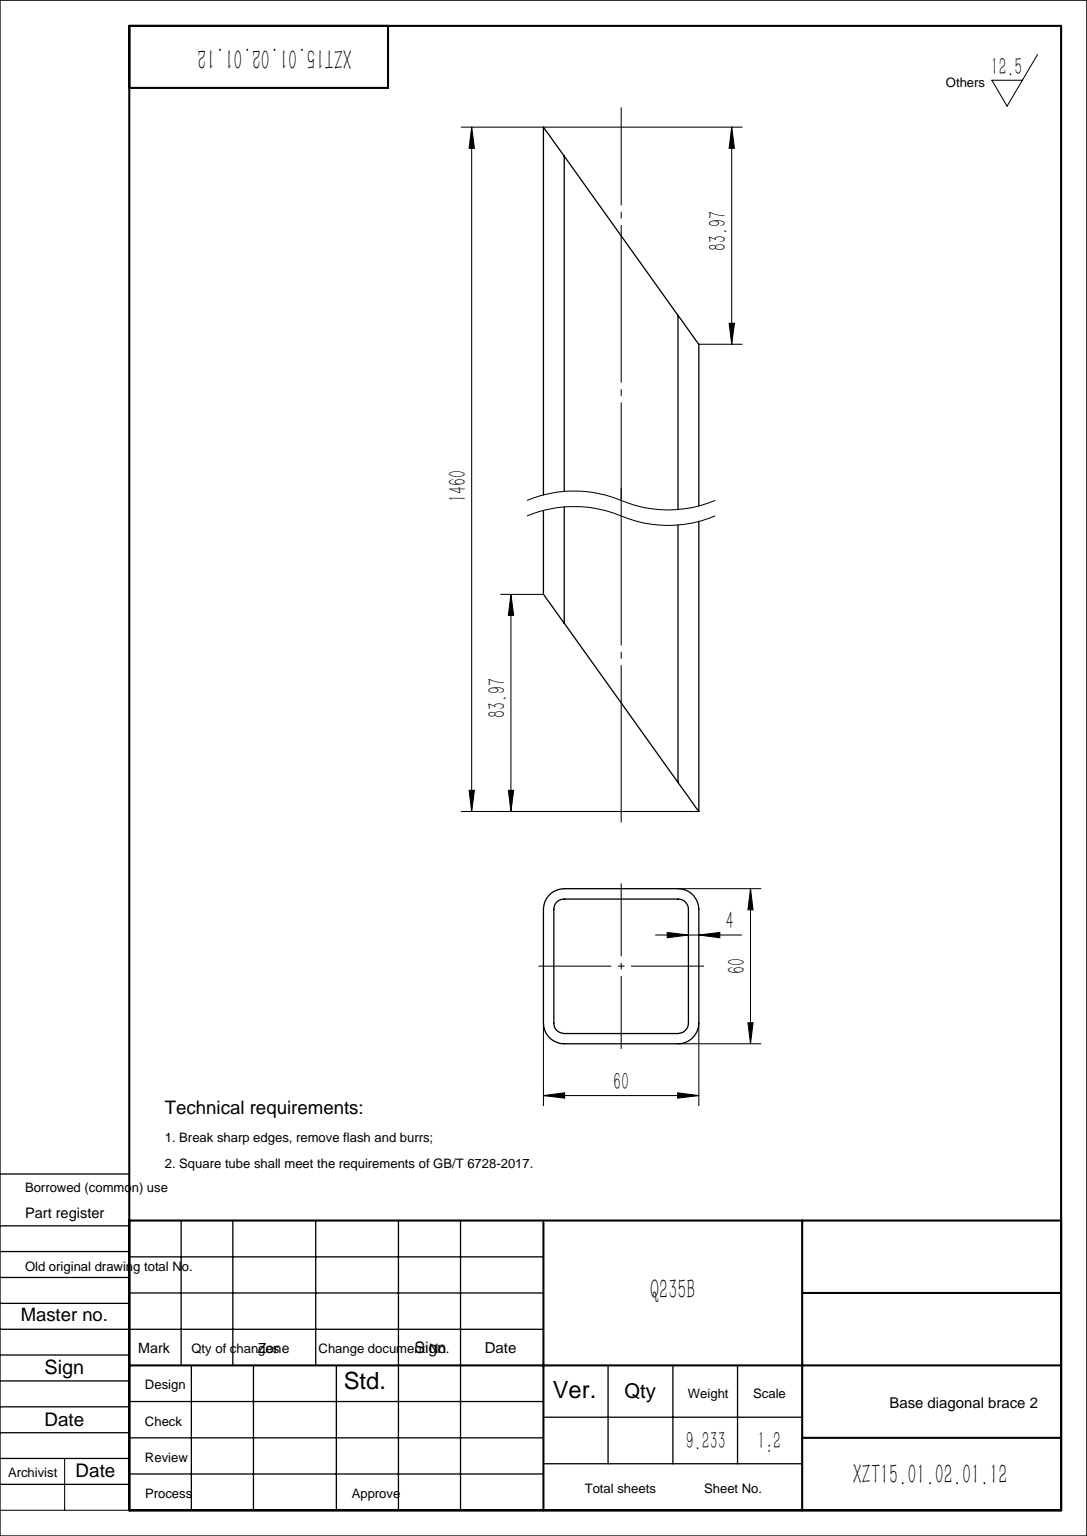
SolidWorks part; units mm, degrees
material "Q235B"
ref_plane "Front Plane" through (0, 0, 0) normal (0, 0, 1) x (1, 0, 0)
ref_plane "Top Plane" through (0, 0, 0) normal (0, 1, 0) x (1, 0, 0)
ref_plane "Right Plane" through (0, 0, 0) normal (1, 0, 0) x (0, 0, -1)
sketch "草图1" plane through (0, 0, 0) normal (0, 0, 1) x (1, 0, 0)
  line L0 (0, 0) -> (0, 1460)
  dimension "D1" = 1460
other "GB/T 6728-2002 square hollow section 60×60×4(1)"
ref_plane "Plane1" through (0, 0, 0) normal (0, 1, 0) x (-1, 0, 0)
sketch "Sketch1" plane through (0, 0, 0) normal (0, 1, 0) x (-1, 0, 0)
  line L0 (-22, -26) -> (22, -26)
  line L1 (-26, -22) -> (-26, 22)
  line L2 (22, 26) -> (-22, 26)
  line L3 (26, 22) -> (26, -22)
  line L4 (-22, -30) -> (22, -30)
  line L5 (-30, -22) -> (-30, 22)
  line L6 (22, 30) -> (-22, 30)
  line L7 (30, 22) -> (30, -22)
  arc A0 (30, 22) -> (22, 30) centre (22, 22) ccw
  arc A1 (22, -30) -> (30, -22) centre (22, -22) ccw
  arc A2 (-30, -22) -> (-22, -30) centre (-22, -22) ccw
  arc A3 (-22, 30) -> (-30, 22) centre (-22, 22) ccw
  arc A4 (-22, 26) -> (-26, 22) centre (-22, 22) ccw
  arc A5 (26, 22) -> (22, 26) centre (22, 22) ccw
  arc A6 (22, -26) -> (26, -22) centre (22, -22) ccw
  arc A7 (-26, -22) -> (-22, -26) centre (-22, -22) ccw
  point P0 (-30, 0)
  point P1 (30, 0)
  point P2 (0, 30)
  point P3 (0, -30)
  point P4 (0, 0)
  point P5 (-30, -30)
  point P6 (30, -30)
  point P7 (30, 30)
  point P8 (-30, 30)
  point P33 (0, 0)
  dimension "D1" = 8
  dimension "Thickness" = 4
  dimension "V_leg" = 60
sketch "Sketch2" plane through (0, 0, 30) normal (0, 0, 1) x (1, 0, 0)
  line L0 (-30, 1460) -> (30, 1376.0314)
  line L1 (30, 1460) -> (30, 0) construction
  line L2 (30, 1376.0314) -> (30, 1460)
  line L3 (30, 1460) -> (-30, 1460)
  line L4 (-30, 0) -> (-30, 83.9686)
  line L5 (-30, 1460) -> (-30, 0) construction
  line L6 (-30, 83.9686) -> (30, 0)
  line L7 (30, 0) -> (-30, 0)
  dimension "D1" = 800
  dimension "D2" = 83.9686
extrude "Cut-Extrude1" cut sketch "Sketch2" against normal through all both and the other way through all
